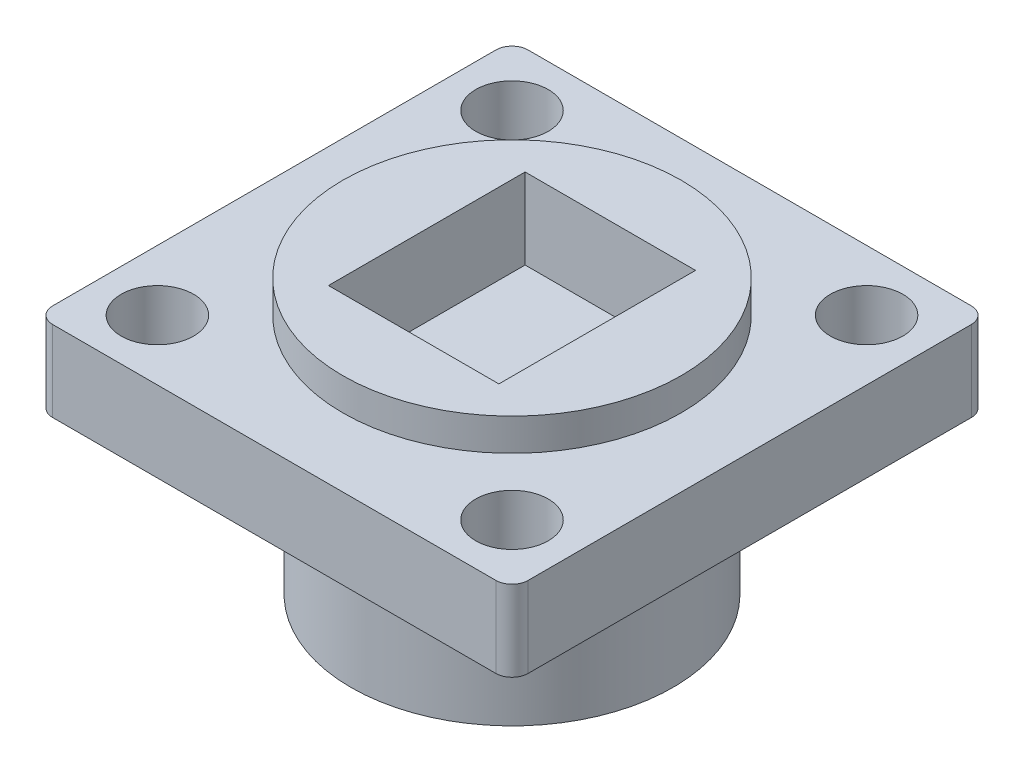
from build123d import *

# Parameters (mm, degrees)
SKETCH_1_R          = 10
EXTRUDE_1_DEPTH     = 10
SKETCH_2_W          = 29.5
SKETCH_2_H          = 29.5
EXTRUDE_2_DEPTH     = 5
SKETCH_3_R          = 10.5
EXTRUDE_3_DEPTH     = 17
SKETCH_4_R          = 2.25
CUT_EXTRUDE_1_DEPTH = 17
FILLET_1_R          = 1
CUT_EXTRUDE_START   = -15
SKETCH_5_R          = 10.5
CUT_EXTRUDE_2_DEPTH = 15
SKETCH_6_W          = 10.574518314
SKETCH_6_H          = 12.201367284
CUT_EXTRUDE_3_DEPTH = 5


with BuildPart() as part:
    # 草图1 → 凸台-拉伸1 (new body)
    with BuildSketch(Plane(origin=(0, 0, 0), x_dir=(1, 0, 0), z_dir=(0, 1, 0))):
        with Locations(Location((0, 0, 0), (0, 0, 270))):
            Circle(SKETCH_1_R)
    extrude(amount=EXTRUDE_1_DEPTH)

    # 草图2 → 凸台-拉伸2 (add)
    with BuildSketch(Plane(origin=(0, 10, 0), x_dir=(1, 0, 0), z_dir=(0, 1, 0))):
        Rectangle(SKETCH_2_W, SKETCH_2_H)
    extrude(amount=EXTRUDE_2_DEPTH)

    # 草图3 → 凸台-拉伸3 (add)
    with BuildSketch(Plane(origin=(0, 15, 0), x_dir=(1, 0, 0), z_dir=(0, 1, 0))):
        with Locations(Location((0, 0, 0), (0, 0, 270))):
            Circle(SKETCH_3_R)
    extrude(amount=EXTRUDE_3_DEPTH)

    # 草图4 → 切除-拉伸1 (cut)
    with BuildSketch(Plane(origin=(0, 15, 0), x_dir=(1, 0, 0), z_dir=(0, 1, 0))):
        with Locations(Location((11, 11, 0), (0, 0, 270))):
            Circle(SKETCH_4_R)
        with Locations(Location((-11, 11, 0), (0, 0, 270))):
            Circle(SKETCH_4_R)
        with Locations(Location((-11, -11, 0), (0, 0, 270))):
            Circle(SKETCH_4_R)
        with Locations(Location((11, -11, 0), (0, 0, 270))):
            Circle(SKETCH_4_R)
    extrude(amount=-CUT_EXTRUDE_1_DEPTH, mode=Mode.SUBTRACT)

    # 圆角1
    fillet_1_edges = [part.edges().sort_by_distance(p)[0] for p in [
        (14.75, 12.5, 14.75),
        (14.75, 12.5, -14.75),
        (-14.75, 12.5, -14.75),
        (-14.75, 12.5, 14.75),
    ]]
    fillet(fillet_1_edges, radius=FILLET_1_R)

    # 草图5 → 切除-拉伸2 (cut)
    with BuildSketch(Plane(origin=(0, 32, 0), x_dir=(1, 0, 0), z_dir=(0, 1, 0)).offset(CUT_EXTRUDE_START)):
        with Locations(Location((0, 0, 0), (0, 0, 270))):
            Circle(SKETCH_5_R)
    extrude(amount=CUT_EXTRUDE_2_DEPTH, mode=Mode.SUBTRACT)

    # 草图6 → 切除-拉伸3 (cut)
    with BuildSketch(Plane(origin=(0, 17, 0), x_dir=(1, 0, 0), z_dir=(0, 1, 0))):
        Rectangle(SKETCH_6_W, SKETCH_6_H)
    extrude(amount=-CUT_EXTRUDE_3_DEPTH, mode=Mode.SUBTRACT)


solid = part.part
